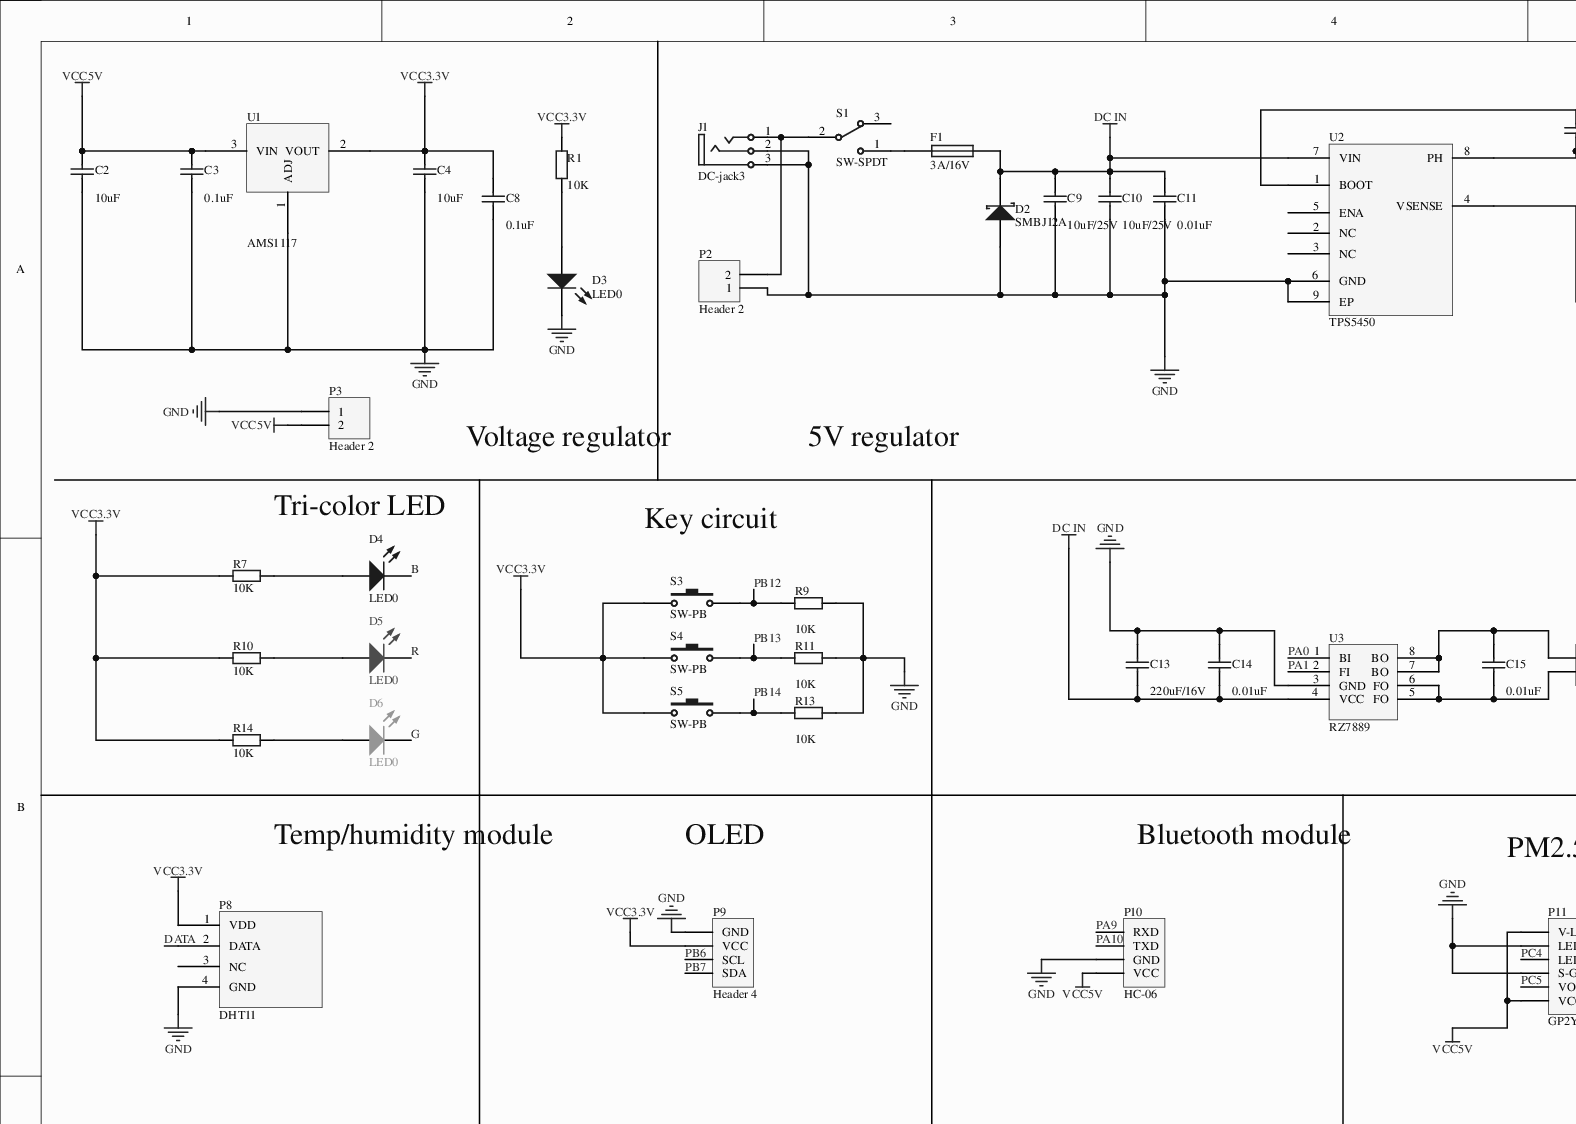
[diagram p0: MISC82341-28.SchDoc, top left]
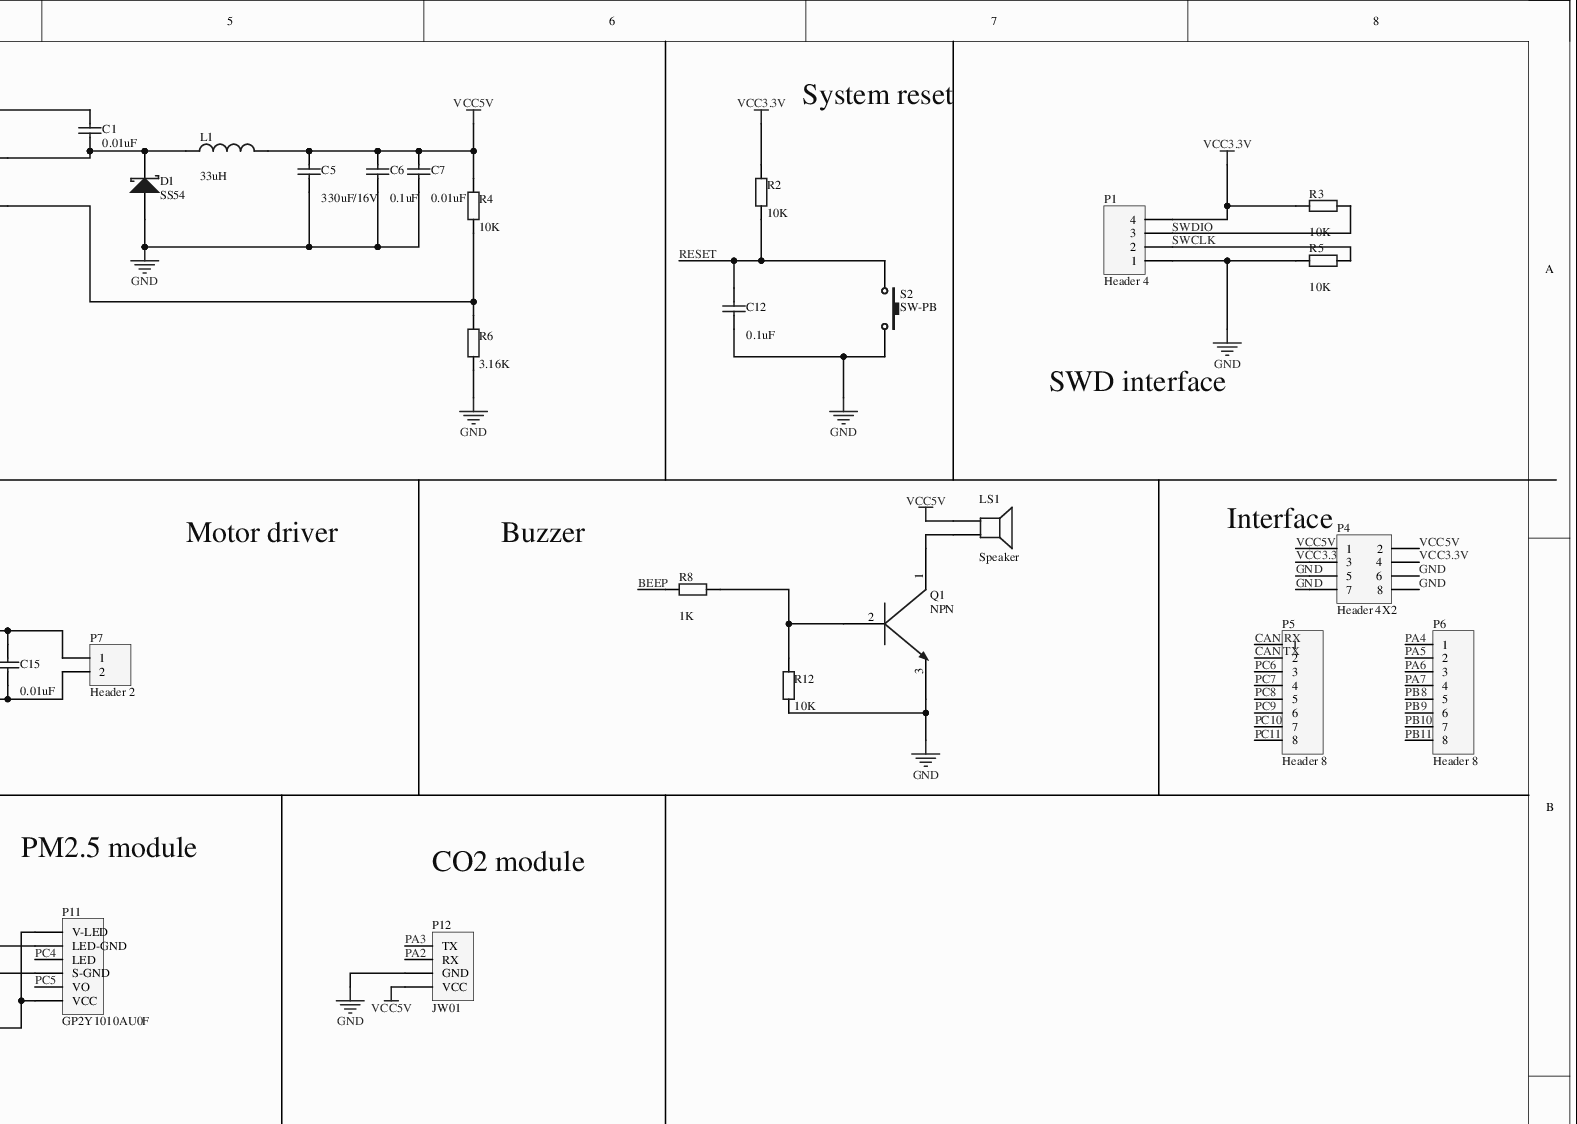
[diagram p1: MISC82341-28.SchDoc, top right]
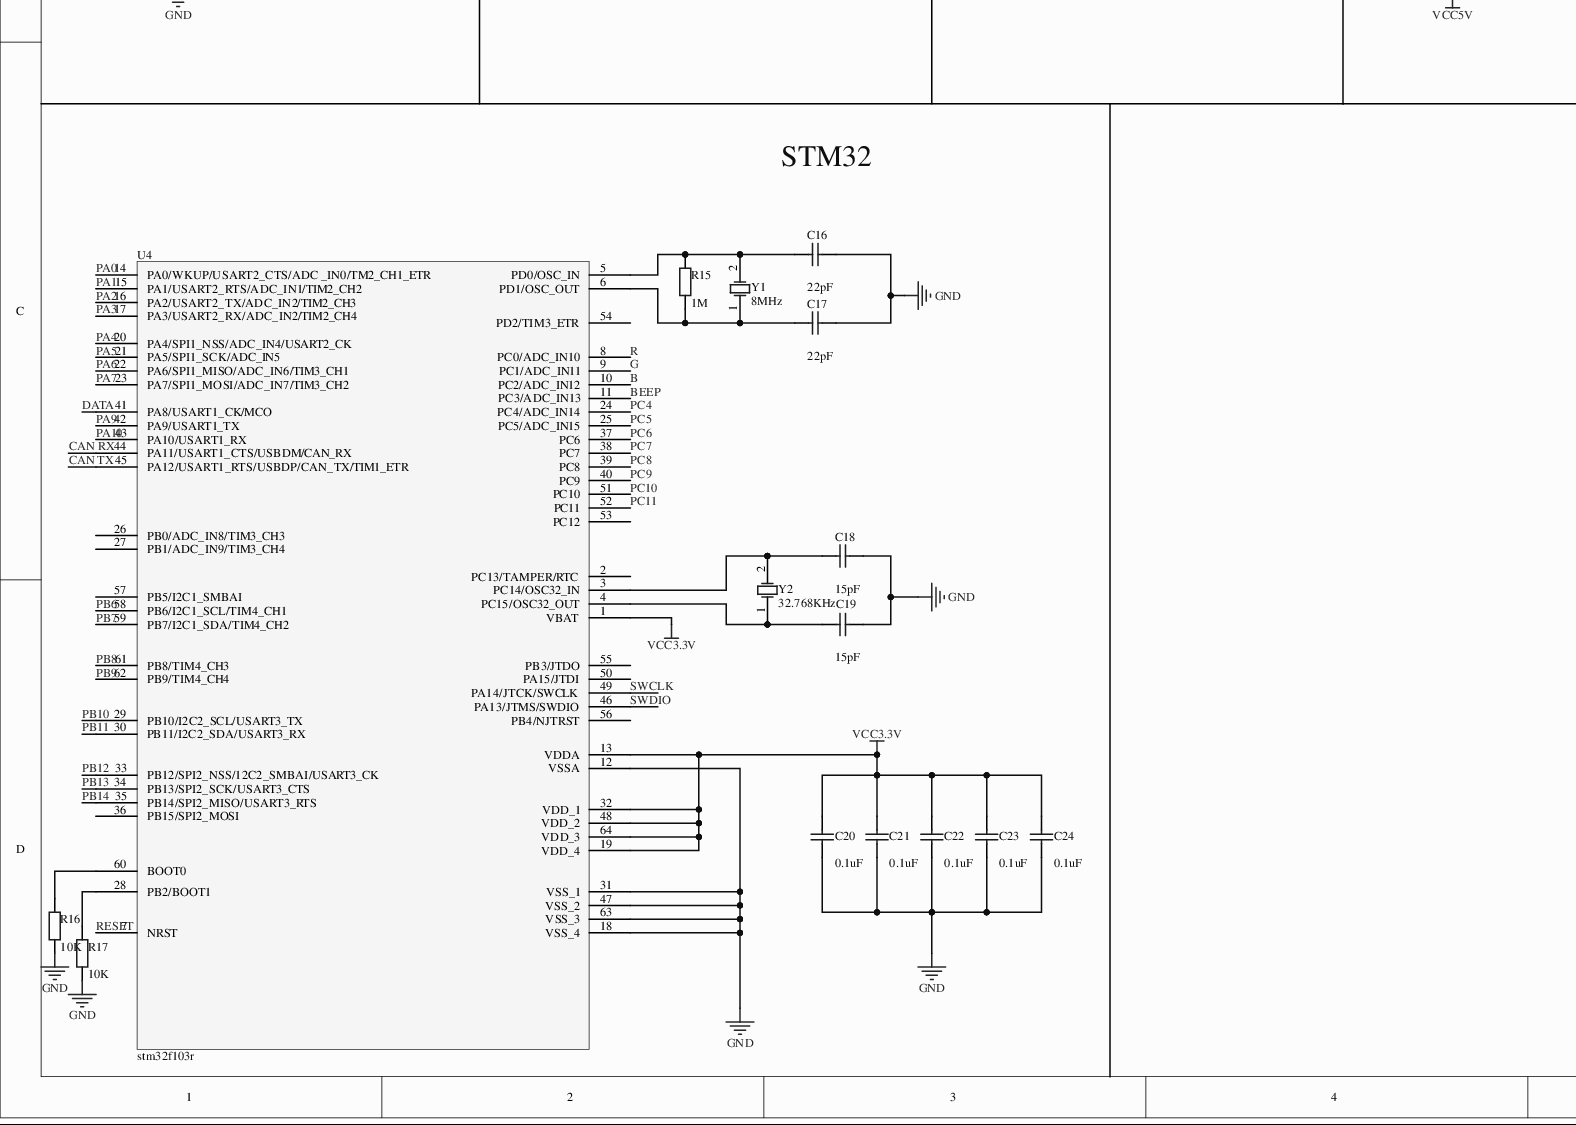
[diagram p2: MISC82341-28.SchDoc, bottom left]
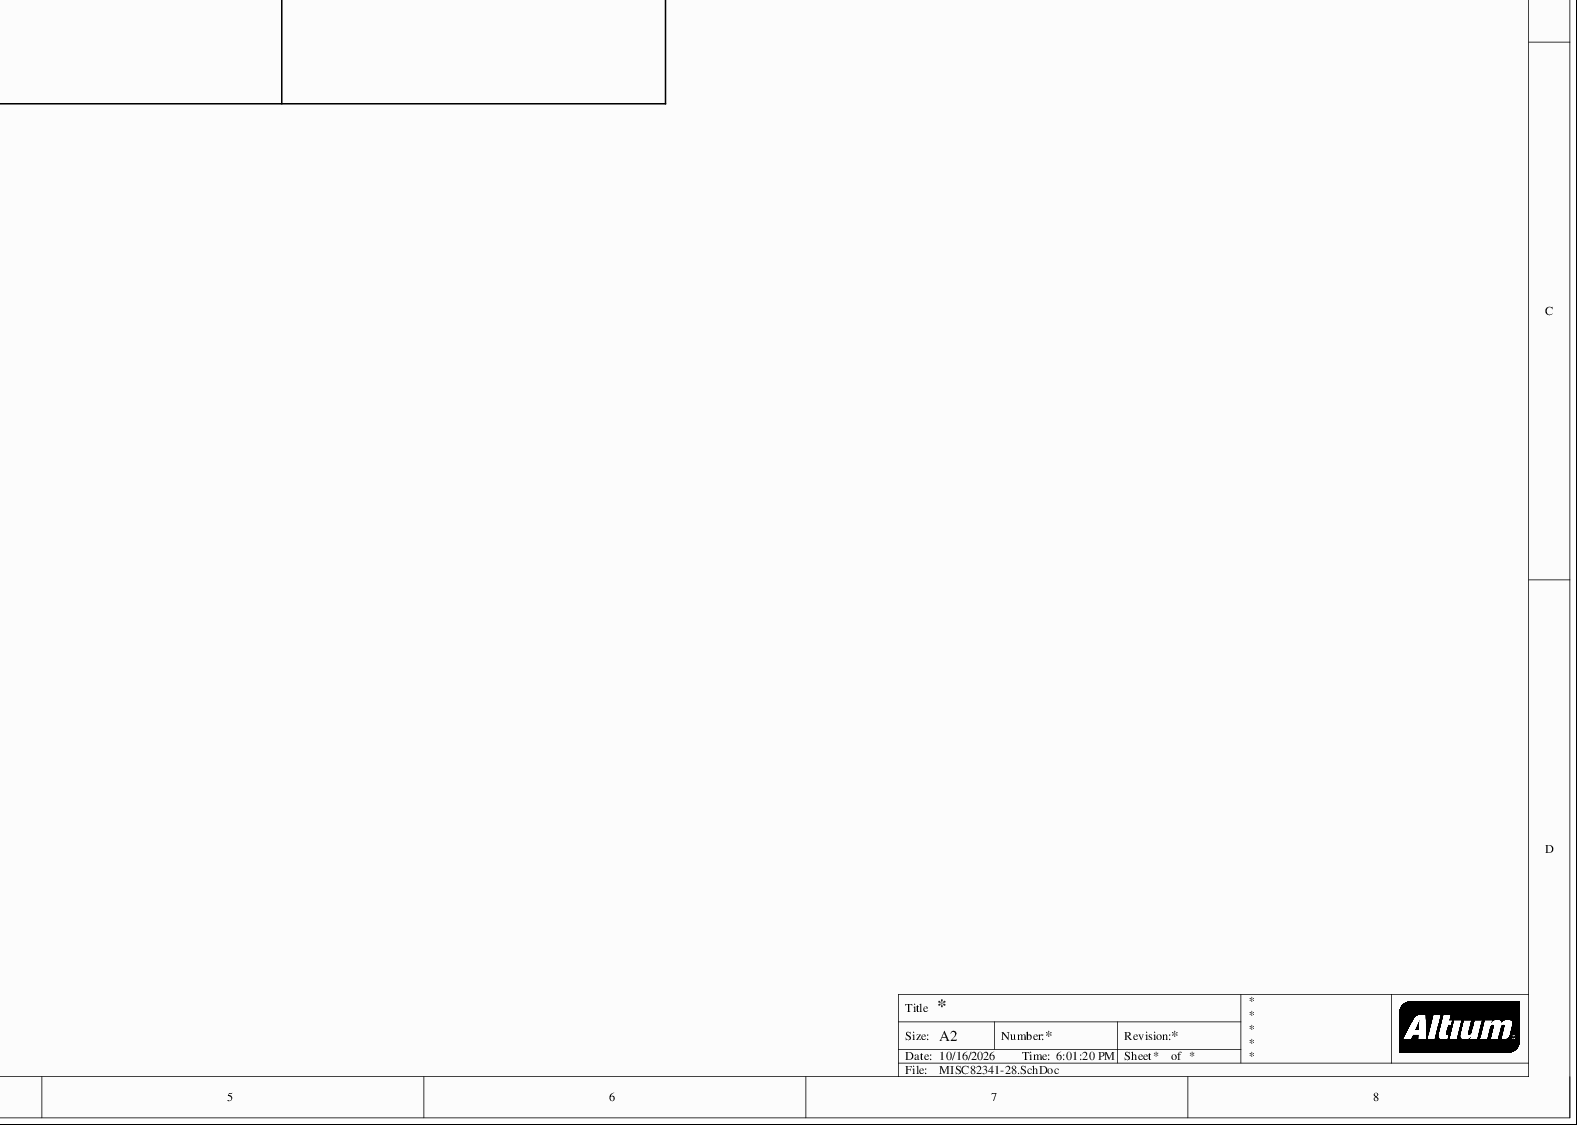
[diagram p3: MISC82341-28.SchDoc, bottom right]
# Altium project MISC82341-9.PrjPcb
1 sheet, 75 parts. Net scope: global (net labels, ports and power ports of the same name join across sheets).
Board file: MISC82341.PcbDoc

## Sheet MISC82341-28.SchDoc
size A2

### Parts
C1  0.01uF  [C0805]
C2  10uF  [C0805]
C3  0.1uF  [C0805]
C4  10uF  [C0805]
C5  330uF/16V  [220uF]
C6  0.1uF  [C0805]
C7  0.01uF  [C0805]
C8  0.1uF  [C0805]
C9  10uF/25V  [C0805]
C10  10uF/25V  [C0805]
C11  0.01uF  [C0805]
C12  0.1uF  [C0805]
C13  220uF/16V  [220uF]
C14  0.01uF  [C0805]
C15  0.01uF  [C0805]
C16  22pF  [C0805]
C17  22pF  [C0805]
C18  15pF  [C0805]
C19  15pF  [C0805]
C20  0.1uF  [C0805]
C21  0.1uF  [C0805]
C22  0.1uF  [C0805]
C23  0.1uF  [C0805]
C24  0.1uF  [C0805]
D1  SS54  [SMA]
D2  SMBJ12A  [SMA]
D3  LED0  [LED0805-RD_RED]
D4  LED0  [LED0805-RD_RED]
D5  LED0  [LED0805-RD_RED]
D6  LED0  [LED0805-RD_RED]
F1  3A/16V  [C70065]
J1  DC-jack3  [SANJIAO]
L1  value 33uH  [DIANGAN]  (hidden comment: Inductor)
LS1  Speaker  [BZ]
P1  Header 4  [HDR1X4]
P2  Header 2  [KF350]
P3  Header 2  [KF350]
P4  Header 4X2  [HDR2X4]
P5  Header 8  [HDR1X8]
P6  Header 8  [HDR1X8]
P7  Header 2  [KF350]
P8  DHT11  [DHT11]
P9  Header 4  [HDR1X4]
P10  HC-06  [HDR1X4]
P11  GP2Y1010AU0F  [HDR1X6]
P12  JW01  [HDR1X4]
Q1  NPN  [QNPN]
R1  10K  [R0805]
R2  10K  [R0805]
R3  10K  [R0805]
R4  10K  [R0805]
R5  10K  [R0805]
R6  3.16K  [R0805]
R7  10K  [R0805]
R8  1K  [R0805]
R9  10K  [R0805]
R10  10K  [R0805]
R11  10K  [R0805]
R12  10K  [R0805]
R13  10K  [R0805]
R14  10K  [R0805]
R15  1M  [R0805]
R16  10K  [R0805]
R17  10K  [R0805]
S1  SW-SPDT  [SW-TH]
S2  SW-PB  [KAIGUAN]
S3  SW-PB  [KAIGUAN]
S4  SW-PB  [KAIGUAN]
S5  SW-PB  [KAIGUAN]
U1  AMS1117  [SOT-89]
U2  TPS5450  [CYF-SOIC-H]
U3  RZ7889  [SOP-8]
U4  stm32f103r  [LQFP-64]
Y1  8MHz  [JINGZHEN]
Y2  32.768KHz  [R38]

### Nets
DC IN: C9.2 C10.2 C11.2 C13.1 C14.1 D2.2(K) F1.2 U2.7(VIN) U3.4(VCC)
GND: C2.1 C3.1 C4.1 C5.1 C6.1 C7.1 C8.1 C9.1 C10.1 C11.1 C12.2 C13.2 C14.2 C16.2 C17.2 C18.1 C19.2 C20.2 C21.2 C22.2 C23.2 C24.2 D1.1(A) D2.1(A) D3.2(K) J1.2(R) J1.3(S) P1.1 P2.1 P3.1 P4.5 P4.6 P4.7 P4.8 P8.4(GND) P9.1(GND) P10.3(GND) P11.2(LED-GND) P11.4(S-GND) P12.3(GND) Q1.3 R5.1 R6.1 R9.2 R11.2 R12.1 R13.2 R16.1 R17.1 S2.2 U1.1(ADJ) U2.6(GND) U2.9(EP) U3.3(GND) U4.12(VSSA) U4.18(VSS_4) U4.31(VSS_1) U4.47(VSS_2) U4.63(VSS_3)
VCC3.3V: C4.2 C8.2 C20.1 C21.1 C22.1 C23.1 C24.1 P1.4 P4.3 P4.4 P8.1(VDD) P9.2(VCC) R1.2 R2.2 R3.1 R7.2 R10.2 R14.2 S3.1 S4.1 S5.1 U1.2(VOUT) U4.1(VBAT) U4.13(VDDA) U4.19(VDD_4) U4.32(VDD_1) U4.48(VDD_2) U4.64(VDD_3)
VCC5V: C2.2 C3.2 C5.2 C6.2 C7.2 L1.2 LS1.1 P3.2 P4.1 P4.2 P10.4(VCC) P11.1(V-LED) P11.6(VCC) P12.4(VCC) R4.2 U1.3(VIN)
B: D4.2(K) U4.10(PC2/ADC_IN12)
BEEP: R8.1 U4.11(PC3/ADC_IN13)
CAN RX: P5.1 U4.44(PA11/USART1_CTS/USBDM/CAN_RX)
CAN TX: P5.2 U4.45(PA12/USART1_RTS/USBDP/CAN_TX/TIM1_ETR)
DATA: P8.2(DATA) U4.41(PA8/USART1_CK/MCO)
G: D6.2(K) U4.9(PC1/ADC_IN11)
PA0: U3.1(BI) U4.14(PA0/WKUP/USART2_CTS/ADC__IN0/TM2_CH1_ETR)
PA1: U3.2(FI) U4.15(PA1/USART2_RTS/ADC_IN1/TIM2_CH2)
PA2: P12.2(RX) U4.16(PA2/USART2_TX/ADC_IN2/TIM2_CH3)
PA3: P12.1(TX) U4.17(PA3/USART2_RX/ADC_IN2/TIM2_CH4)
PA4: P6.1 U4.20(PA4/SPI1_NSS/ADC_IN4/USART2_CK)
PA5: P6.2 U4.21(PA5/SPI1_SCK/ADC_IN5)
PA6: P6.3 U4.22(PA6/SPI1_MISO/ADC_IN6/TIM3_CH1)
PA7: P6.4 U4.23(PA7/SPI1_MOSI/ADC_IN7/TIM3_CH2)
PA9: P10.1(RXD) U4.42(PA9/USART1_TX)
PA10: P10.2(TXD) U4.43(PA10/USART1_RX)
PB6: P9.3(SCL) U4.58(PB6/I2C1_SCL/TIM4_CH1)
PB7: P9.4(SDA) U4.59(PB7/I2C1_SDA/TIM4_CH2)
PB8: P6.5 U4.61(PB8/TIM4_CH3)
PB9: P6.6 U4.62(PB9/TIM4_CH4)
PB10: P6.7 U4.29(PB10/I2C2_SCL/USART3_TX)
PB11: P6.8 U4.30(PB11/I2C2_SDA/USART3_RX)
PB12: R9.1 S3.2 U4.33(PB12/SPI2_NSS/12C2_SMBAI/USART3_CK)
PB13: R11.1 S4.2 U4.34(PB13/SPI2_SCK/USART3_CTS)
PB14: R13.1 S5.2 U4.35(PB14/SPI2_MISO/USART3_RTS)
PC4: P11.3(LED) U4.24(PC4/ADC_IN14)
PC5: P11.5(VO) U4.25(PC5/ADC_IN15)
PC6: P5.3 U4.37(PC6)
PC7: P5.4 U4.38(PC7)
PC8: P5.5 U4.39(PC8)
PC9: P5.6 U4.40(PC9)
PC10: P5.7 U4.51(PC10)
PC11: P5.8 U4.52(PC11)
R: D5.2(K) U4.8(PC0/ADC_IN10)
RESET: C12.1 R2.1 S2.1 U4.7(NRST)
SWCLK: P1.2 R5.2 U4.49(PA14/JTCK/SWCLK)
SWDIO: P1.3 R3.2 U4.46(PA13/JTMS/SWDIO)
NetC1_1: C1.1 U2.1(BOOT)
NetC1_2: C1.2 D1.2(K) L1.1 U2.8(PH)
NetC15_1: C15.1 P7.2 U3.5(FO) U3.6(FO)
NetC15_2: C15.2 P7.1 U3.7(BO) U3.8(BO)
NetC16_1: C16.1 R15.2 U4.5(PD0/OSC_IN) Y1.2(OSC2)
NetC17_1: C17.1 R15.1 U4.6(PD1/OSC_OUT) Y1.1(OSC1)
NetC18_2: C18.2 U4.3(PC14/OSC32_IN) Y2.2(OSC2)
NetC19_1: C19.1 U4.4(PC15/OSC32_OUT) Y2.1(OSC1)
NetD3_1: D3.1(A) R1.1
NetD4_1: D4.1(A) R7.1
NetD5_1: D5.1(A) R10.1
NetD6_1: D6.1(A) R14.1
NetF1_1: F1.1 S1.1
NetJ1_1: J1.1(T) P2.2 S1.2
NetLS1_2: LS1.2 Q1.1
NetQ1_2: Q1.2 R8.2 R12.2
NetR4_1: R4.1 R6.2 U2.4(VSENSE)
NetR16_2: R16.2 U4.60(BOOT0)
NetR17_2: R17.2 U4.28(PB2/BOOT1)

Not connected (* = marked no-connect by the designer): P8 3(NC)*; S1 3*; U2 2(NC) 3(NC) 5(ENA); U4 2(PC13/TAMPER/RTC) 26(PB0/ADC_IN8/TIM3_CH3) 27(PB1/ADC_IN9/TIM3_CH4) 36(PB15/SPI2_MOSI) 50(PA15/JTDI)* 53(PC12) 54(PD2/TIM3_ETR) 55(PB3/JTDO)* 56(PB4/NJTRST) 57(PB5/I2C1_SMBAI)

### Notes on the sheet
- System reset
- SWD interface
- Voltage regulator
- 5V regulator
- Tri-color LED
- Key circuit
- (near P4) Interface
- Motor driver
- Buzzer
- Temp/humidity module
- OLED
- Bluetooth module
- PM2.5 module
- CO2 module
- STM32
- Title
- Size:
- Date:
- File:
- A2
- Number:
- Time:
- Revision:
- Sheet
- of

### Library data of the parts
C1-C24 = Cap: Capacitor; Published: 8-Jun-2000; LatestRevisionDate: 17-Jul-2002; LatestRevisionNote: Re-released for DXP Platform.; PackageReference: RAD-0.3; PackageDescription: Radial Cap, Thru-Hole; 2 Leads; 0.3 in Pin Spacing; Publisher: Altium Limited
  C1 C7 C11 C14 C15: Value: 0.01uF
  C2 C4: Value: 10uF
  C3 C6 C8 C12 C20-C24: Value: 0.1uF
  C5: Value: 330uF/16V
  C9 C10: Value: 10uF/25V
  C13: Value: 220uF/16V
  C16 C17: Value: 22pF
  C18 C19: Value: 15pF
D1 D2 = D Schottky: Schottky Diode; Published: 8-Jun-2000; LatestRevisionDate: 17-Jul-2002; LatestRevisionNote: Re-released for DXP Platform.; PackageReference: SMB; PackageDescription: DO-214-AA/SMB; 2 C-Bend Leads; Body 5.3 x 3.6 mm, inc. leads (LxW); Code_JEDEC: DO-214-AA; Publisher: Altium Limited
D3-D6 = LED0: Typical INFRARED GaAs LED; Published: 8-Jun-2000; LatestRevisionDate: 08-Jul-2005; LatestRevisionNote: Mech Layer 1 removed.; PackageReference: LED-0; PackageDescription: LED; 2 Leads; Publisher: Altium Limited
F1 = Fuse 1: Fuse; Published: 8-Jun-2000; LatestRevisionDate: 17-Jul-2002; LatestRevisionNote: Re-released for DXP Platform.; PackageReference: PIN-W2/E2.8; PackageDescription: Thru-Hole; 2 Leads; Publisher: Altium Limited
L1 = Inductor: Code_IEC: 1005; Published: 8-Jun-2000; LatestRevisionDate: 29-May-2009; LatestRevisionNote: IPC-7351 Footprint Added.; PackageReference: 0402-A; PackageDescription: Chip Inductor; Code_JEITA: 0402; Publisher: Altium Limited
LS1 = Speaker: Loudspeaker; Published: 24-Mar-1999; LatestRevisionDate: 17-Jul-2002; LatestRevisionNote: Re-released for DXP Platform.; PackageReference: PIN2; Publisher: Altium Limited
P1 P9 P10 P12 = Header 4: Header, 4-Pin; LatestRevisionDate: 17-Jul-2002; LatestRevisionNote: Re-released for DXP Platform.; Publisher: Altium Limited
P2 P3 P7 = Header 2: Header, 2-Pin; LatestRevisionDate: 17-Jul-2002; LatestRevisionNote: Re-released for DXP Platform.; Publisher: Altium Limited
P4 = Header 4X2: Header, 4-Pin, Dual row; LatestRevisionDate: 17-Jul-2002; LatestRevisionNote: Re-released for DXP Platform.; Publisher: Altium Limited
P5 P6 = Header 8: Header, 8-Pin; LatestRevisionDate: 17-Jul-2002; LatestRevisionNote: Re-released for DXP Platform.; Publisher: Altium Limited
P11 = Header 6: Header, 6-Pin; LatestRevisionDate: 17-Jul-2002; LatestRevisionNote: Re-released for DXP Platform.; Publisher: Altium Limited
R1-R17 = Res2: Resistor; Published: 8-Jun-2000; LatestRevisionDate: 17-Jul-2002; LatestRevisionNote: Re-released for DXP Platform.; PackageReference: AXIAL-0.4; PackageDescription: Axial Device, Thru-Hole; 2 Leads; 0.4 in Pin Spacing; Publisher: Altium Limited
  R1-R5 R7 R9-R14 R16 R17: Value: 10K
  R6: Value: 3.16K
  R8: Value: 1K
  R15: Value: 1M
S1 = SW-SPDT: SPDT Subminiature Toggle Switch, Right Angle Mounting, Vertical Actuation; Published: 24-Mar-1999; LatestRevisionDate: 17-Dec-2003; LatestRevisionNote: Schematic revised, PCB Footprint replaced.; DatasheetVersion: 05-Dec-2000; PackageReference: TL36WW15050; PackageDescription: Switch; 4 Leads; ComponentLink1Description: Manufacturer Link; Publisher: Altium Limited
S2-S5 = SW-PB: Switch; Published: 24-Mar-1999; LatestRevisionDate: 17-Jul-2002; LatestRevisionNote: Re-released for DXP Platform.; PackageReference: SPST-2; PackageDescription: Switch; 2 Leads; Publisher: Altium Limited
Y1 Y2 = XTAL: Crystal Oscillator; Published: 8-Jun-2000; LatestRevisionDate: 17-Jul-2002; LatestRevisionNote: Re-released for DXP Platform.; PackageReference: R38; PackageDescription: Crystal, Thru-Hole; 2 Leads; Body 3.1 x 8.2 mm (Dia.xH); Publisher: Altium Limited